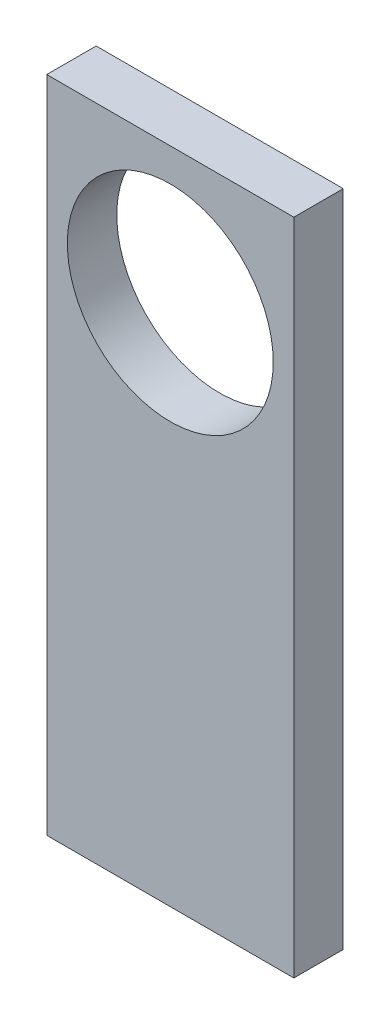
from build123d import *

# Parameters (mm, degrees)
SKETCH_1_W          = 60
SKETCH_1_H          = 160
EXTRUDE_1_DEPTH     = 12
SKETCH_2_R          = 25
CUT_EXTRUDE_1_DEPTH = 87.27861844


with BuildPart() as part:
    # 草图1 → 凸台-拉伸1 (new body)
    with BuildSketch(Plane.XY):
        Rectangle(SKETCH_1_W, SKETCH_1_H)
    extrude(amount=EXTRUDE_1_DEPTH)

    # 草图2 → 切除-拉伸1 (cut, through all)
    with BuildSketch(Plane.XY.offset(12)):
        with Locations((0, 47)):
            Circle(SKETCH_2_R)
    extrude(amount=-CUT_EXTRUDE_1_DEPTH, mode=Mode.SUBTRACT)


solid = part.part
